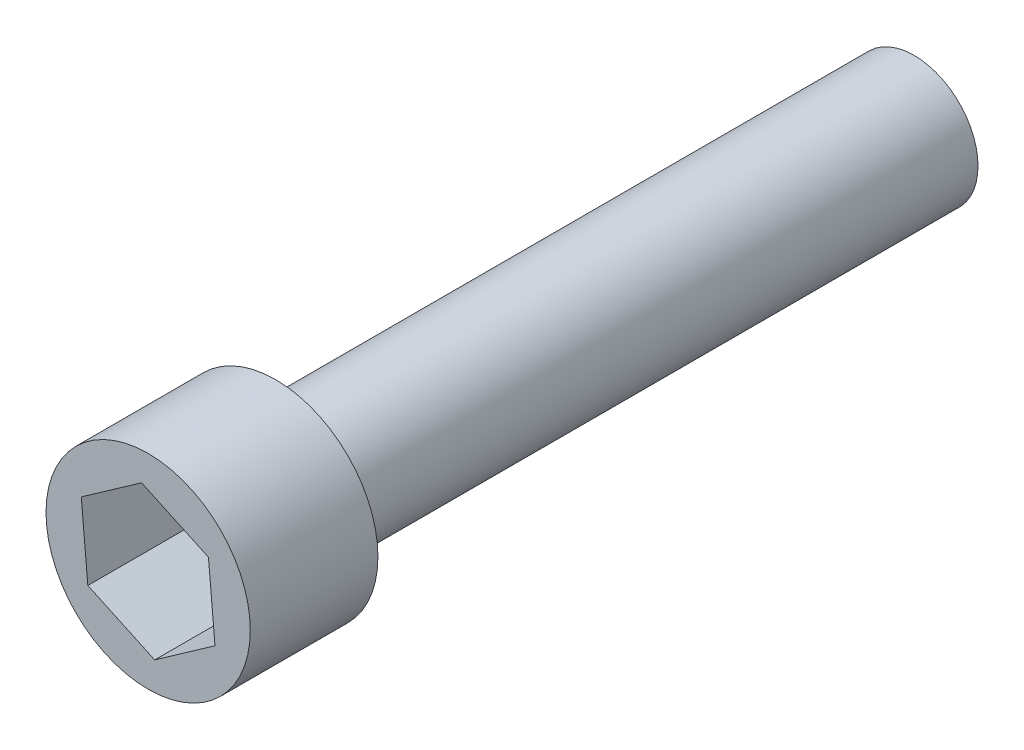
SolidWorks part; units mm, degrees
ref_plane "Front Plane" through (0, 0, 0) normal (0, 0, 1) x (1, 0, 0)
ref_plane "Top Plane" through (0, 0, 0) normal (0, 1, 0) x (1, 0, 0)
ref_plane "Right Plane" through (0, 0, 0) normal (1, 0, 0) x (0, 0, -1)
sketch "Sketch1" plane through (0, 0, 0) normal (0, 0, 1) x (1, 0, 0)
  circle A0 centre (0, 0) radius 5
  dimension "D1" = 10
extrude "Boss-Extrude1" add sketch "Sketch1" along normal blind 50
sketch "Sketch2" plane through (0, 0, 50) normal (0, 0, 1) x (1, 0, 0)
  circle A0 centre (0, 0) radius 8
  dimension "D1" = 16
extrude "Boss-Extrude2" add sketch "Sketch2" along normal blind 10
sketch "Sketch3" plane through (0, 0, 60) normal (0, 0, 1) x (1, 0, 0)
  line L1 (0.5141, -5.7506) -> (5.2372, -2.43)
  line L2 (5.2372, -2.43) -> (4.7231, 3.3205)
  line L3 (4.7231, 3.3205) -> (-0.5141, 5.7506)
  line L4 (-0.5141, 5.7506) -> (-5.2372, 2.43)
  line L5 (-5.2372, 2.43) -> (-4.7231, -3.3205)
  line L6 (-4.7231, -3.3205) -> (0.5141, -5.7506)
  circle A0 centre (0, 0) radius 5 construction
  dimension "D1" = 10
extrude "Cut-Extrude1" cut sketch "Sketch3" against normal blind 8
